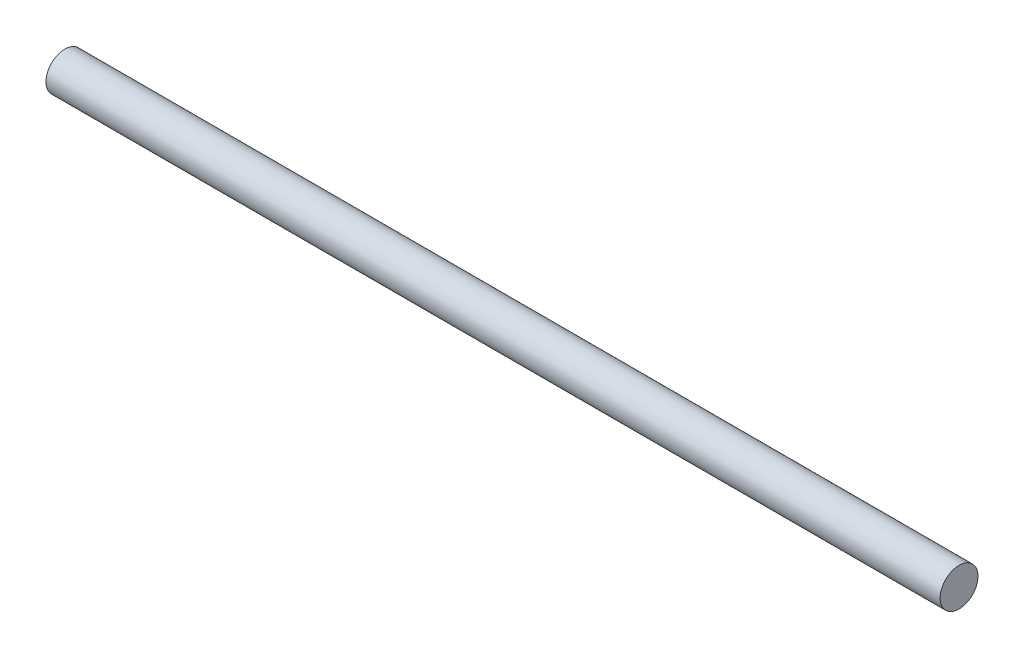
SolidWorks part; units mm, degrees
material "不锈钢201"
ref_plane "前视基准面" through (0, 0, 0) normal (0, 0, 1) x (1, 0, 0)
ref_plane "上视基准面" through (0, 0, 0) normal (0, 1, 0) x (1, 0, 0)
ref_plane "右视基准面" through (0, 0, 0) normal (1, 0, 0) x (0, 0, -1)
sketch "草图1" plane through (0, 0, 0) normal (1, 0, 0) x (0, 0, -1)
  circle A0 centre (0, 0) radius 2.5
  dimension "D1" = 5
extrude "凸台-拉伸1" add sketch "草图1" along normal blind 118
